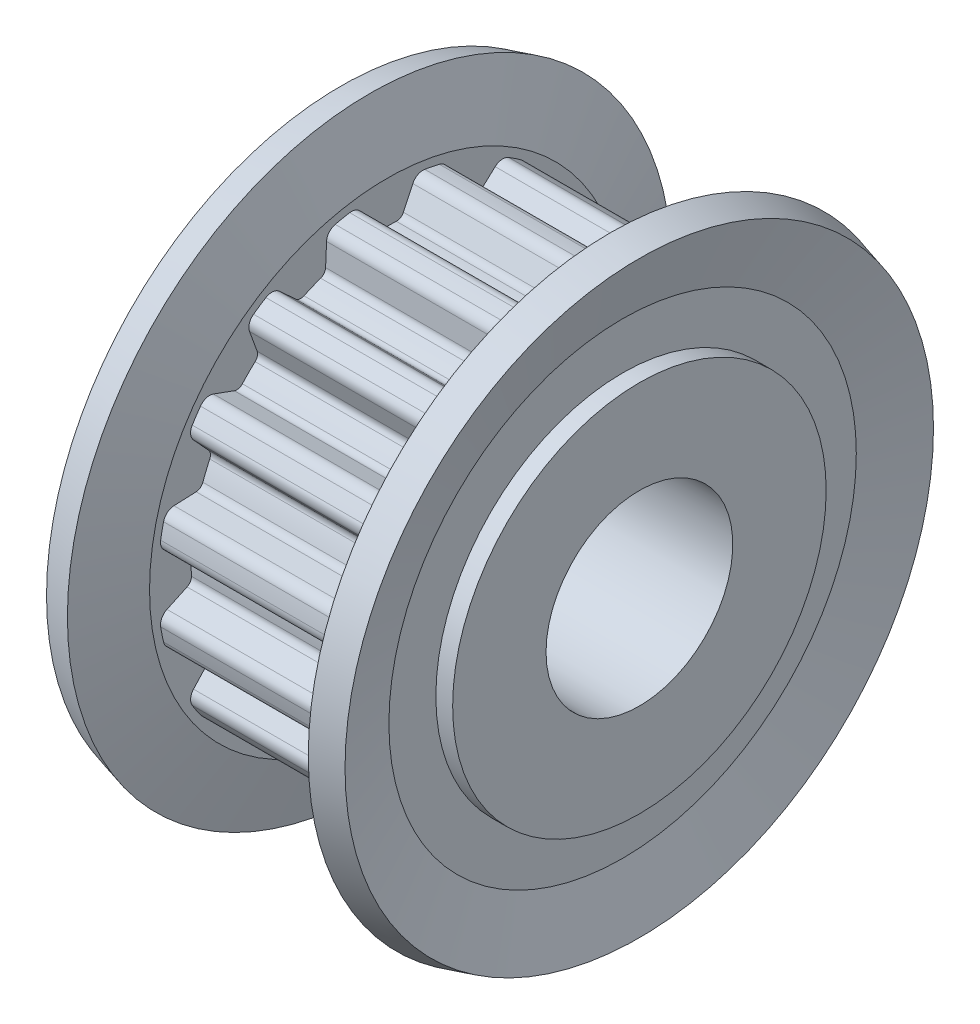
from build123d import *

# Parameters (mm, degrees)
SKETCH_2_W          = 64
SKETCH_2_H          = 64
CUT_EXTRUDE_1_DEPTH = 11


with BuildPart() as part:
    # 草图1 → 旋转1 (revolve)
    with BuildSketch(Plane.XY, mode=Mode.PRIVATE) as revolve_1_sk:
        Polygon((0, 9.8), (0, 5.2), (0.2, 5), (16, 5), (16, 10), (15.1, 10), (15.1, 12.513835473), (15.991930053, 15.754514664), (14.449291918, 16.179093968), (13.5, 12.73), (2.5, 12.73), (1.550708082, 16.179093968), (0.008069947, 15.754514664), (0.9, 12.513835473), (0.9, 10), (0.2, 10), align=None)
    revolve(revolve_1_sk.sketch.rotate(Axis((28, 0, 0), (-1, 0, 0)), 270), axis=Axis((28, 0, 0), (-1, 0, 0)))

    # 草图2 → 切除-拉伸1 (cut)
    with BuildSketch(Plane(origin=(2.5, 0, 0), x_dir=(0, 0, -1), z_dir=(1, 0, 0))):
        Rectangle(SKETCH_2_W, SKETCH_2_H)
        with BuildLine():
            Line((-11.421675295, -3.251314352), (-10.234355553, -3.303153851))
            ThreePointArc((-10.234355553, -3.303153851), (-10.014882256, -3.380486909), (-9.875590343, -3.566891557))
            ThreePointArc((-9.875590343, -3.566891557), (-9.700735091, -4.01817604), (-9.505270107, -4.460923692))
            ThreePointArc((-9.505270107, -4.460923692), (-9.471956373, -4.691225939), (-9.5724647, -4.901099725))
            Line((-9.5724647, -4.901099725), (-10.37537048, -5.777317628))
            ThreePointArc((-10.37537048, -5.777317628), (-10.530438739, -6.127247702), (-10.442388892, -6.499731859))
            ThreePointArc((-10.442388892, -6.499731859), (-10.336079998, -6.667492053), (-10.227076231, -6.833513866))
            ThreePointArc((-10.227076231, -6.833513866), (-10.115406006, -6.997754021), (-10.001098443, -7.160169686))
            ThreePointArc((-10.001098443, -7.160169686), (-9.690663174, -7.38406064), (-9.308027896, -7.374708689))
            Line((-9.308027896, -7.374708689), (-8.191249371, -6.968234547))
            ThreePointArc((-8.191249371, -6.968234547), (-7.958888404, -6.955692181), (-7.758865485, -7.074602913))
            ThreePointArc((-7.758865485, -7.074602913), (-7.424621202, -7.424621202), (-7.074602913, -7.758865485))
            ThreePointArc((-7.074602913, -7.758865485), (-6.955692181, -7.958888404), (-6.968234547, -8.191249371))
            Line((-6.968234547, -8.191249371), (-7.374708689, -9.308027896))
            ThreePointArc((-7.374708689, -9.308027896), (-7.384060643, -9.690663165), (-7.160169702, -10.001098431))
            ThreePointArc((-7.160169702, -10.001098431), (-6.997754029, -10.115406), (-6.833513866, -10.227076231))
            ThreePointArc((-6.833513866, -10.227076231), (-6.667492045, -10.336080003), (-6.499731842, -10.442388902))
            ThreePointArc((-6.499731842, -10.442388902), (-6.127247693, -10.530438738), (-5.777317628, -10.37537048))
            Line((-5.777317628, -10.37537048), (-4.901099725, -9.5724647))
            ThreePointArc((-4.901099725, -9.5724647), (-4.691225939, -9.471956373), (-4.460923692, -9.505270107))
            ThreePointArc((-4.460923692, -9.505270107), (-4.01817604, -9.700735091), (-3.566891557, -9.875590343))
            ThreePointArc((-3.566891557, -9.875590343), (-3.380486909, -10.014882256), (-3.303153851, -10.234355553))
            Line((-3.303153851, -10.234355553), (-3.251314352, -11.421675295))
            ThreePointArc((-3.251314352, -11.421675295), (-3.113526253, -11.778763026), (-2.787879562, -11.979888461))
            ThreePointArc((-2.787879562, -11.979888461), (-2.594083433, -12.023341097), (-2.399610961, -12.063658949))
            ThreePointArc((-2.399610961, -12.063658949), (-2.20451286, -12.100831502), (-2.008839989, -12.134849068))
            ThreePointArc((-2.008839989, -12.134849068), (-1.631014293, -12.073652996), (-1.367063122, -11.796476168))
            Line((-1.367063122, -11.796476168), (-0.864802075, -10.719373878))
            ThreePointArc((-0.864802075, -10.719373878), (-0.709366852, -10.54620107), (-0.483846705, -10.488846093))
            ThreePointArc((-0.483846705, -10.488846093), (0, -10.5), (0.483846705, -10.488846093))
            ThreePointArc((0.483846705, -10.488846093), (0.709366852, -10.54620107), (0.864802075, -10.719373878))
            Line((0.864802075, -10.719373878), (1.367063122, -11.796476168))
            ThreePointArc((1.367063122, -11.796476168), (1.631014267, -12.073652983), (2.00883993, -12.134849078))
            ThreePointArc((2.00883993, -12.134849078), (2.204512831, -12.100831508), (2.399610961, -12.063658949))
            ThreePointArc((2.399610961, -12.063658949), (2.594083423, -12.023341099), (2.787879543, -11.979888466))
            ThreePointArc((2.787879543, -11.979888466), (3.113526247, -11.778763034), (3.251314352, -11.421675295))
            Line((3.251314352, -11.421675295), (3.303153851, -10.234355553))
            ThreePointArc((3.303153851, -10.234355553), (3.380486909, -10.014882256), (3.566891557, -9.875590343))
            ThreePointArc((3.566891557, -9.875590343), (4.01817604, -9.700735091), (4.460923692, -9.505270107))
            ThreePointArc((4.460923692, -9.505270107), (4.691225939, -9.471956373), (4.901099725, -9.5724647))
            Line((4.901099725, -9.5724647), (5.777317628, -10.37537048))
            ThreePointArc((5.777317628, -10.37537048), (6.127247683, -10.530438737), (6.499731825, -10.442388912))
            ThreePointArc((6.499731825, -10.442388912), (6.667492036, -10.336080009), (6.833513866, -10.227076231))
            ThreePointArc((6.833513866, -10.227076231), (6.997754021, -10.115406006), (7.160169686, -10.001098443))
            ThreePointArc((7.160169686, -10.001098443), (7.38406064, -9.690663174), (7.374708689, -9.308027896))
            Line((7.374708689, -9.308027896), (6.968234547, -8.191249371))
            ThreePointArc((6.968234547, -8.191249371), (6.955692181, -7.958888404), (7.074602913, -7.758865485))
            ThreePointArc((7.074602913, -7.758865485), (7.424621202, -7.424621202), (7.758865485, -7.074602913))
            ThreePointArc((7.758865485, -7.074602913), (7.958888404, -6.955692181), (8.191249371, -6.968234547))
            Line((8.191249371, -6.968234547), (9.308027896, -7.374708689))
            ThreePointArc((9.308027896, -7.374708689), (9.690663165, -7.384060643), (10.001098431, -7.160169702))
            ThreePointArc((10.001098431, -7.160169702), (10.115406, -6.997754029), (10.227076231, -6.833513866))
            ThreePointArc((10.227076231, -6.833513866), (10.336080003, -6.667492045), (10.442388902, -6.499731842))
            ThreePointArc((10.442388902, -6.499731842), (10.530438738, -6.127247693), (10.37537048, -5.777317628))
            Line((10.37537048, -5.777317628), (9.5724647, -4.901099725))
            ThreePointArc((9.5724647, -4.901099725), (9.471956373, -4.691225939), (9.505270107, -4.460923692))
            ThreePointArc((9.505270107, -4.460923692), (9.700735091, -4.01817604), (9.875590343, -3.566891557))
            ThreePointArc((9.875590343, -3.566891557), (10.014882256, -3.380486909), (10.234355553, -3.303153851))
            Line((10.234355553, -3.303153851), (11.421675295, -3.251314352))
            ThreePointArc((11.421675295, -3.251314352), (11.778763026, -3.113526253), (11.979888461, -2.787879562))
            ThreePointArc((11.979888461, -2.787879562), (12.023341097, -2.594083433), (12.063658949, -2.399610961))
            ThreePointArc((12.063658949, -2.399610961), (12.100831502, -2.20451286), (12.134849068, -2.008839989))
            ThreePointArc((12.134849068, -2.008839989), (12.073652996, -1.631014293), (11.796476168, -1.367063122))
            Line((11.796476168, -1.367063122), (10.719373878, -0.864802075))
            ThreePointArc((10.719373878, -0.864802075), (10.54620107, -0.709366852), (10.488846093, -0.483846705))
            ThreePointArc((10.488846093, -0.483846705), (10.5, 0), (10.488846093, 0.483846705))
            ThreePointArc((10.488846093, 0.483846705), (10.54620107, 0.709366852), (10.719373878, 0.864802075))
            Line((10.719373878, 0.864802075), (11.796476168, 1.367063122))
            ThreePointArc((11.796476168, 1.367063122), (12.073652983, 1.631014267), (12.134849078, 2.00883993))
            ThreePointArc((12.134849078, 2.00883993), (12.100831508, 2.204512831), (12.063658949, 2.399610961))
            ThreePointArc((12.063658949, 2.399610961), (12.023341099, 2.594083423), (11.979888466, 2.787879543))
            ThreePointArc((11.979888466, 2.787879543), (11.778763034, 3.113526247), (11.421675295, 3.251314352))
            Line((11.421675295, 3.251314352), (10.234355553, 3.303153851))
            ThreePointArc((10.234355553, 3.303153851), (10.014882256, 3.380486909), (9.875590343, 3.566891557))
            ThreePointArc((9.875590343, 3.566891557), (9.700735091, 4.01817604), (9.505270107, 4.460923692))
            ThreePointArc((9.505270107, 4.460923692), (9.471956373, 4.691225939), (9.5724647, 4.901099725))
            Line((9.5724647, 4.901099725), (10.37537048, 5.777317628))
            ThreePointArc((10.37537048, 5.777317628), (10.530438737, 6.127247683), (10.442388912, 6.499731825))
            ThreePointArc((10.442388912, 6.499731825), (10.336080009, 6.667492036), (10.227076231, 6.833513866))
            ThreePointArc((10.227076231, 6.833513866), (10.115406006, 6.997754021), (10.001098443, 7.160169686))
            ThreePointArc((10.001098443, 7.160169686), (9.690663174, 7.38406064), (9.308027896, 7.374708689))
            Line((9.308027896, 7.374708689), (8.191249371, 6.968234547))
            ThreePointArc((8.191249371, 6.968234547), (7.958888404, 6.955692181), (7.758865485, 7.074602913))
            ThreePointArc((7.758865485, 7.074602913), (7.424621202, 7.424621202), (7.074602913, 7.758865485))
            ThreePointArc((7.074602913, 7.758865485), (6.955692181, 7.958888404), (6.968234547, 8.191249371))
            Line((6.968234547, 8.191249371), (7.374708689, 9.308027896))
            ThreePointArc((7.374708689, 9.308027896), (7.384060643, 9.690663165), (7.160169702, 10.001098431))
            ThreePointArc((7.160169702, 10.001098431), (6.997754029, 10.115406), (6.833513866, 10.227076231))
            ThreePointArc((6.833513866, 10.227076231), (6.667492045, 10.336080003), (6.499731842, 10.442388902))
            ThreePointArc((6.499731842, 10.442388902), (6.127247693, 10.530438738), (5.777317628, 10.37537048))
            Line((5.777317628, 10.37537048), (4.901099725, 9.5724647))
            ThreePointArc((4.901099725, 9.5724647), (4.691225939, 9.471956373), (4.460923692, 9.505270107))
            ThreePointArc((4.460923692, 9.505270107), (4.01817604, 9.700735091), (3.566891557, 9.875590343))
            ThreePointArc((3.566891557, 9.875590343), (3.380486909, 10.014882256), (3.303153851, 10.234355553))
            Line((3.303153851, 10.234355553), (3.251314352, 11.421675295))
            ThreePointArc((3.251314352, 11.421675295), (3.113526253, 11.778763026), (2.787879562, 11.979888461))
            ThreePointArc((2.787879562, 11.979888461), (2.594083433, 12.023341097), (2.399610961, 12.063658949))
            ThreePointArc((2.399610961, 12.063658949), (2.20451286, 12.100831502), (2.008839989, 12.134849068))
            ThreePointArc((2.008839989, 12.134849068), (1.631014293, 12.073652996), (1.367063122, 11.796476168))
            Line((1.367063122, 11.796476168), (0.864802075, 10.719373878))
            ThreePointArc((0.864802075, 10.719373878), (0.709366852, 10.54620107), (0.483846705, 10.488846093))
            ThreePointArc((0.483846705, 10.488846093), (0, 10.5), (-0.483846705, 10.488846093))
            ThreePointArc((-0.483846705, 10.488846093), (-0.709366852, 10.54620107), (-0.864802075, 10.719373878))
            Line((-0.864802075, 10.719373878), (-1.367063122, 11.796476168))
            ThreePointArc((-1.367063122, 11.796476168), (-1.631014285, 12.073652992), (-2.008839969, 12.134849071))
            ThreePointArc((-2.008839969, 12.134849071), (-2.204512851, 12.100831504), (-2.399610961, 12.063658949))
            ThreePointArc((-2.399610961, 12.063658949), (-2.594083423, 12.0233411), (-2.787879543, 11.979888466))
            ThreePointArc((-2.787879543, 11.979888466), (-3.113526247, 11.778763034), (-3.251314352, 11.421675295))
            Line((-3.251314352, 11.421675295), (-3.303153851, 10.234355553))
            ThreePointArc((-3.303153851, 10.234355553), (-3.380486909, 10.014882256), (-3.566891557, 9.875590343))
            ThreePointArc((-3.566891557, 9.875590343), (-4.01817604, 9.700735091), (-4.460923692, 9.505270107))
            ThreePointArc((-4.460923692, 9.505270107), (-4.691225939, 9.471956373), (-4.901099725, 9.5724647))
            Line((-4.901099725, 9.5724647), (-5.777317628, 10.37537048))
            ThreePointArc((-5.777317628, 10.37537048), (-6.127247683, 10.530438737), (-6.499731825, 10.442388912))
            ThreePointArc((-6.499731825, 10.442388912), (-6.667492036, 10.336080009), (-6.833513866, 10.227076231))
            ThreePointArc((-6.833513866, 10.227076231), (-6.997754021, 10.115406006), (-7.160169686, 10.001098443))
            ThreePointArc((-7.160169686, 10.001098443), (-7.38406064, 9.690663175), (-7.374708689, 9.308027896))
            Line((-7.374708689, 9.308027896), (-6.968234547, 8.191249371))
            ThreePointArc((-6.968234547, 8.191249371), (-6.955692181, 7.958888404), (-7.074602913, 7.758865485))
            ThreePointArc((-7.074602913, 7.758865485), (-7.424621202, 7.424621202), (-7.758865485, 7.074602913))
            ThreePointArc((-7.758865485, 7.074602913), (-7.958888404, 6.955692181), (-8.191249371, 6.968234547))
            Line((-8.191249371, 6.968234547), (-9.308027896, 7.374708689))
            ThreePointArc((-9.308027896, 7.374708689), (-9.690663174, 7.38406064), (-10.001098443, 7.160169686))
            ThreePointArc((-10.001098443, 7.160169686), (-10.115406006, 6.997754021), (-10.227076231, 6.833513866))
            ThreePointArc((-10.227076231, 6.833513866), (-10.336080003, 6.667492045), (-10.442388902, 6.499731842))
            ThreePointArc((-10.442388902, 6.499731842), (-10.530438738, 6.127247693), (-10.37537048, 5.777317628))
            Line((-10.37537048, 5.777317628), (-9.5724647, 4.901099725))
            ThreePointArc((-9.5724647, 4.901099725), (-9.471956373, 4.691225939), (-9.505270107, 4.460923692))
            ThreePointArc((-9.505270107, 4.460923692), (-9.700735091, 4.01817604), (-9.875590343, 3.566891557))
            ThreePointArc((-9.875590343, 3.566891557), (-10.014882256, 3.380486909), (-10.234355553, 3.303153851))
            Line((-10.234355553, 3.303153851), (-11.421675295, 3.251314352))
            ThreePointArc((-11.421675295, 3.251314352), (-11.778763042, 3.113526241), (-11.97988847, 2.787879524))
            ThreePointArc((-11.97988847, 2.787879524), (-12.023341102, 2.594083413), (-12.063658949, 2.399610961))
            ThreePointArc((-12.063658949, 2.399610961), (-12.100831502, 2.20451286), (-12.134849068, 2.008839989))
            ThreePointArc((-12.134849068, 2.008839989), (-12.073652996, 1.631014293), (-11.796476168, 1.367063122))
            Line((-11.796476168, 1.367063122), (-10.719373878, 0.864802075))
            ThreePointArc((-10.719373878, 0.864802075), (-10.54620107, 0.709366852), (-10.488846093, 0.483846705))
            ThreePointArc((-10.488846093, 0.483846705), (-10.5, 0), (-10.488846093, -0.483846705))
            ThreePointArc((-10.488846093, -0.483846705), (-10.54620107, -0.709366852), (-10.719373878, -0.864802075))
            Line((-10.719373878, -0.864802075), (-11.796476168, -1.367063122))
            ThreePointArc((-11.796476168, -1.367063122), (-12.073653001, -1.631014302), (-12.134849065, -2.008840008))
            ThreePointArc((-12.134849065, -2.008840008), (-12.100831501, -2.20451287), (-12.063658949, -2.399610961))
            ThreePointArc((-12.063658949, -2.399610961), (-12.023341099, -2.594083423), (-11.979888466, -2.787879543))
            ThreePointArc((-11.979888466, -2.787879543), (-11.778763034, -3.113526247), (-11.421675295, -3.251314352))
        make_face(mode=Mode.SUBTRACT)
    extrude(amount=CUT_EXTRUDE_1_DEPTH, mode=Mode.SUBTRACT)


solid = part.part
